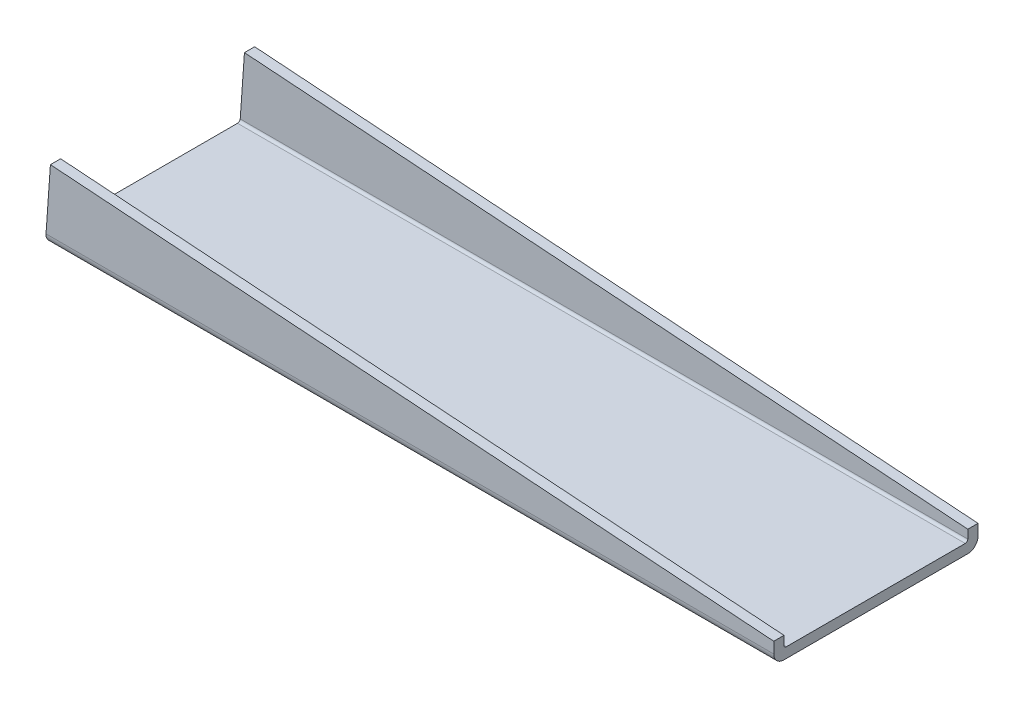
SolidWorks part; units mm, degrees
material "1023 碳钢板 (SS)"
ref_plane "前视基准面" through (0, 0, 0) normal (0, 0, 1) x (1, 0, 0)
ref_plane "上视基准面" through (0, 0, 0) normal (0, 1, 0) x (1, 0, 0)
ref_plane "右视基准面" through (0, 0, 0) normal (1, 0, 0) x (0, 0, -1)
sketch "草图1" plane through (0, 0, 0) normal (0, 0, 1) x (1, 0, 0)
  line L1 (425, 42.5) -> (-425, 42.5)
  line L2 (425, 42.5) -> (425, -42.5)
  line L3 (425, -42.5) -> (-425, -42.5)
  line L4 (-425, 42.5) -> (-425, -42.5)
  line L5 (425, 42.5) -> (-425, -42.5) construction
  line L6 (425, -42.5) -> (-425, 42.5) construction
  point P0 (0, 0)
  dimension "D1" = 850
  dimension "D2" = 85
extrude "凸台-拉伸1" add sketch "草图1" along normal blind 240
sketch "草图2" plane through (0, 0, 240) normal (0, 0, 1) x (1, 0, 0)
  line L0 (-425, 42.5) -> (425, -17.5)
  line L1 (425, -42.5) -> (425, 42.5) construction
  line L2 (-425, 42.5) -> (425, 42.5)
  line L3 (425, 42.5) -> (425, -17.5)
  dimension "D1" = 25
extrude "切除-拉伸1" cut sketch "草图2" against normal blind 240
shell "抽壳1" thickness 12
sketch "草图6" plane through (0, 0, 0) normal (0, 0, -1) x (-1, 0, 0)
  line L1 (425, 42.5) -> (431, -42.5)
  line L2 (431, -42.5) -> (425, -42.5)
  line L3 (425, -42.5) -> (425, 42.5)
extrude "凸台-拉伸2" add sketch "草图6" against normal blind 240
sketch "草图5" plane through (0, -30.5, 0) normal (0, 1, 0) x (1, 0, 0)
  line L4 (425, -12) -> (-425, -12)
  line L5 (-425, -12) -> (-425, -228)
  line L6 (-425, -228) -> (425, -228)
  line L7 (425, -228) -> (425, -12)
  line L8 (425, -12) -> (-425, -12)
  line L10 (-425, -228) -> (425, -228)
  line L11 (425, -228) -> (425, -12)
  line L12 (-425, -12) -> (-425, -228)
  dimension "D1" = 0
extrude "切除-拉伸3" cut sketch "草图5" along normal blind 94
fillet "圆角1" radius 12 2 edges at (-3, -42.5, 240) (-3, -42.5, 0)
fillet "圆角2" radius 3 2 edges at (0, -30.5, 12) (0, -30.5, 228)
sketch "草图7" plane through (-425, 0, 0) normal (1, 0, 0) x (0, 0, -1)
  line L4 (-225, -30.5) -> (-15, -30.5)
  line L5 (-12, -27.5) -> (-12, 42.5)
  line L6 (-12, 42.5) -> (-228, 42.5)
  line L7 (-228, 42.5) -> (-228, -27.5)
  line L8 (-225, -30.5) -> (-15, -30.5)
  line L9 (-12, -27.5) -> (-12, 42.5)
  line L10 (-12, 42.5) -> (-228, 42.5)
  line L11 (-228, 42.5) -> (-228, -27.5)
  arc A2 (-15, -30.5) -> (-12, -27.5) centre (-15, -27.5) ccw
  arc A3 (-228, -27.5) -> (-225, -30.5) centre (-225, -27.5) ccw
  arc A4 (-15, -30.5) -> (-12, -27.5) centre (-15, -27.5) ccw
  arc A5 (-228, -27.5) -> (-225, -30.5) centre (-225, -27.5) ccw
  dimension "D1" = 0
extrude "切除-拉伸4" cut sketch "草图7" against normal blind 240
